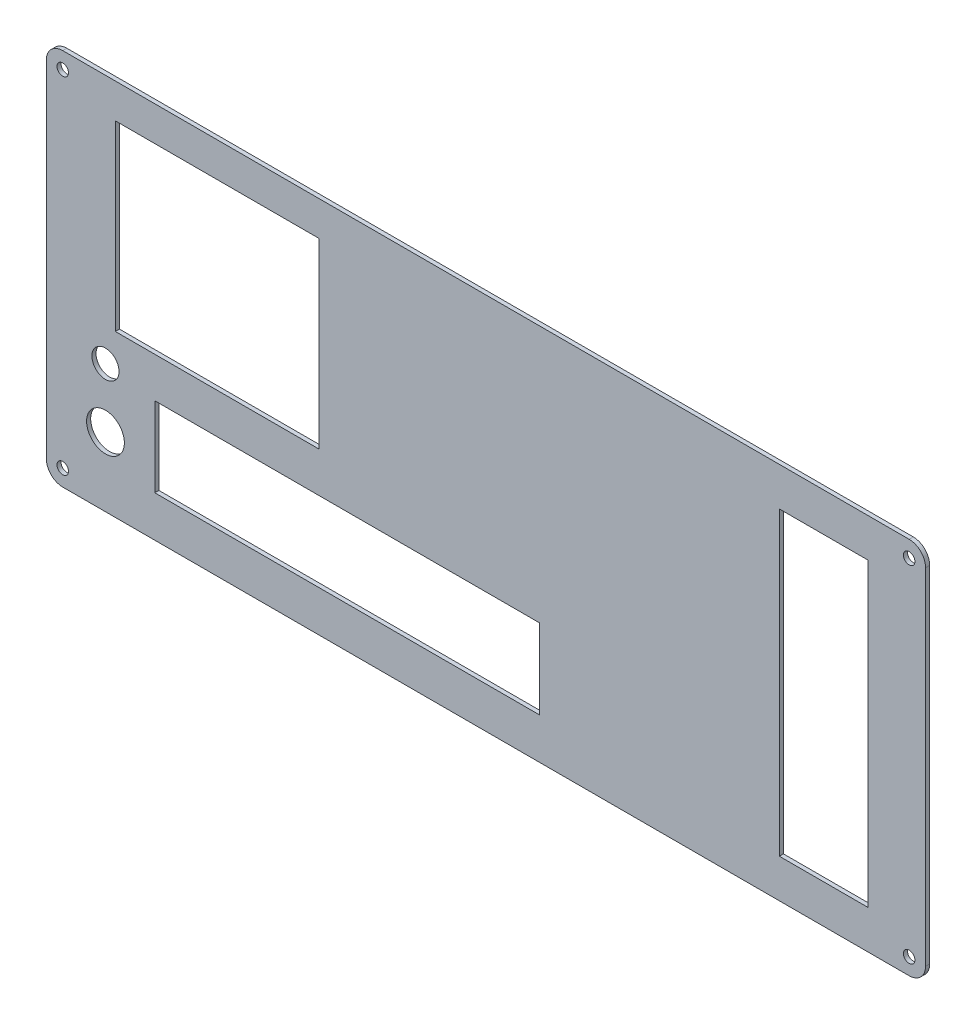
from build123d import *

# Parameters (mm, degrees)
SKETCH1_W            = 535
SKETCH1_H            = 230
BOSS_EXTRUDE1_DEPTH  = 2.5
FILLET1_R            = 10
SKETCH2_R            = 3.5
CUT_EXTRUDE1_DEPTH   = 2.5
LPATTERN1_COUNT      = 2
LPATTERN1_PITCH      = 515
LPATTERN1_COUNT_DIR2 = 2
LPATTERN1_PITCH_DIR2 = 210
SKETCH3_W            = 124
SKETCH3_H            = 111
CUT_EXTRUDE2_DEPTH   = 2.5
SKETCH4_W            = 234
SKETCH4_H            = 48.5
CUT_EXTRUDE3_DEPTH   = 2.5
SKETCH5_R            = 11.5
CUT_EXTRUDE4_DEPTH   = 2.5
SKETCH7_R            = 8.25
CUT_EXTRUDE5_DEPTH   = 2.5
SKETCH8_W            = 54
SKETCH8_H            = 183
CUT_EXTRUDE6_DEPTH   = 2.5


with BuildPart() as part:
    # Sketch1 → Boss-Extrude1 (new body)
    with BuildSketch(Plane.XY):
        with Locations((267.5, -115)):
            Rectangle(SKETCH1_W, SKETCH1_H)
    extrude(amount=BOSS_EXTRUDE1_DEPTH)

    # Fillet1
    fillet1_edges = [part.edges().sort_by_distance(p)[0] for p in [
        (0, 0, 1.25),
        (535, 0, 1.25),
        (535, -230, 1.25),
        (0, -230, 1.25),
    ]]
    fillet(fillet1_edges, radius=FILLET1_R)

    # Sketch2 → Cut-Extrude1 (cut)
    with BuildSketch(Plane.XY.offset(2.5)):
        with Locations((10, -10)):
            Circle(SKETCH2_R)
    cut_extrude1 = extrude(amount=-CUT_EXTRUDE1_DEPTH, mode=Mode.SUBTRACT)

    # LPattern1: Cut-Extrude1 2 × 2
    with Locations(*[(i * LPATTERN1_PITCH, -j * LPATTERN1_PITCH_DIR2, 0) for i in range(LPATTERN1_COUNT) for j in range(LPATTERN1_COUNT_DIR2) if (i, j) != (0, 0)]):
        add(cut_extrude1, mode=Mode.SUBTRACT)

    # Sketch3 → Cut-Extrude2 (cut)
    with BuildSketch(Plane.XY.offset(2.5)):
        with Locations((104, -76.5)):
            Rectangle(SKETCH3_W, SKETCH3_H)
    extrude(amount=-CUT_EXTRUDE2_DEPTH, mode=Mode.SUBTRACT)

    # Sketch4 → Cut-Extrude3 (cut)
    with BuildSketch(Plane.XY.offset(2.5)):
        with Locations((183, -180.75)):
            Rectangle(SKETCH4_W, SKETCH4_H)
    extrude(amount=-CUT_EXTRUDE3_DEPTH, mode=Mode.SUBTRACT)

    # Sketch5 → Cut-Extrude4 (cut)
    with BuildSketch(Plane.XY.offset(2.5)):
        with Locations((36, -188)):
            Circle(SKETCH5_R)
    extrude(amount=-CUT_EXTRUDE4_DEPTH, mode=Mode.SUBTRACT)

    # Sketch7 → Cut-Extrude5 (cut)
    with BuildSketch(Plane.XY.offset(2.5)):
        with Locations((36, -152)):
            Circle(SKETCH7_R)
    extrude(amount=-CUT_EXTRUDE5_DEPTH, mode=Mode.SUBTRACT)

    # Sketch8 → Cut-Extrude6 (cut)
    with BuildSketch(Plane.XY.offset(2.5)):
        with Locations((473, -115)):
            Rectangle(SKETCH8_W, SKETCH8_H)
    extrude(amount=-CUT_EXTRUDE6_DEPTH, mode=Mode.SUBTRACT)


solid = part.part
